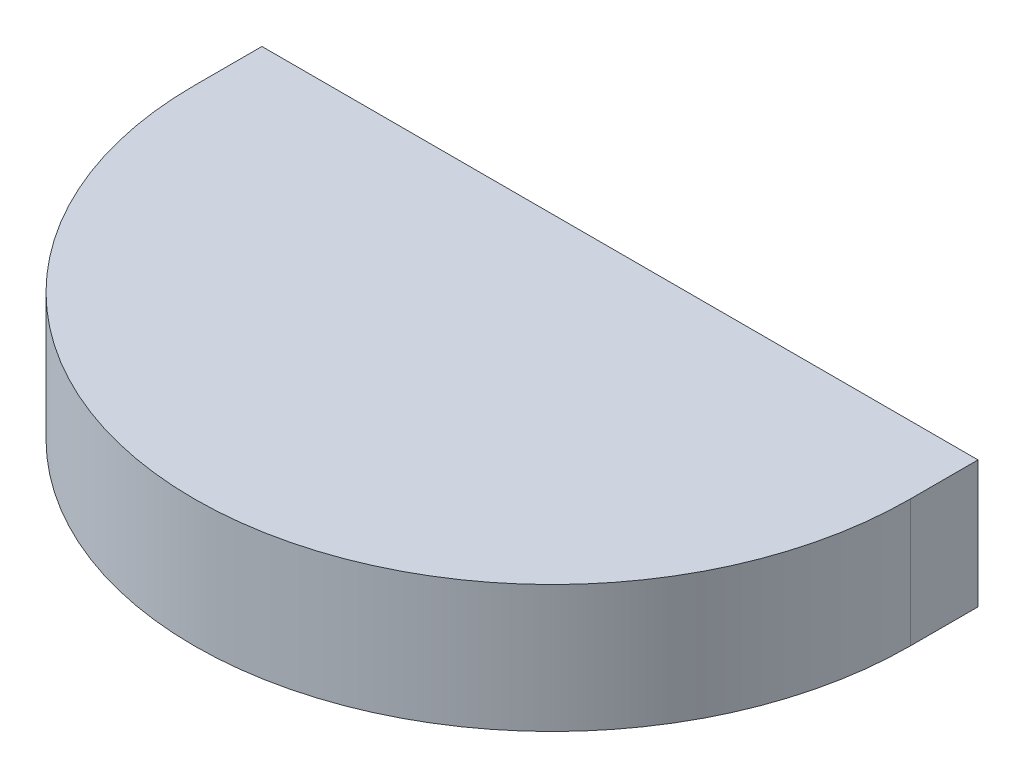
SolidWorks part; units mm, degrees
ref_plane "Front Plane" through (0, 0, 0) normal (0, 0, 1) x (1, 0, 0)
ref_plane "Top Plane" through (0, 0, 0) normal (0, 1, 0) x (1, 0, 0)
ref_plane "Right Plane" through (0, 0, 0) normal (1, 0, 0) x (0, 0, -1)
sketch "Sketch1" plane through (0, 0, 0) normal (0, 1, 0) x (1, 0, 0)
  line L1 (-27.1288, 0) -> (-27.1288, 1.7)
  line L2 (-27.1288, 1.7) -> (-9.1288, 1.7)
  line L3 (-9.1288, 1.7) -> (-9.1288, 0)
  arc A0 (-27.1288, 0) -> (-9.1288, 0) centre (-18.1288, 0) ccw
  dimension "D1" = 18
  dimension "D2" = 1.7
extrude "Extrude1" add sketch "Sketch1" along normal blind 3.2
